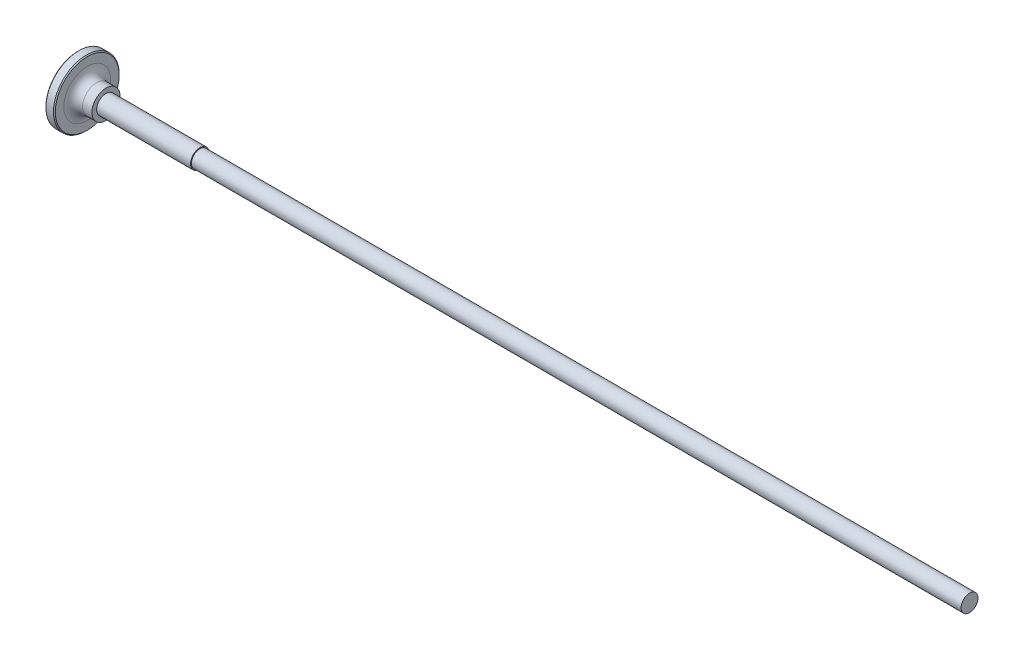
SolidWorks part; units mm, degrees
ref_plane "前视基准面" through (0, 0, 0) normal (0, 0, 1) x (1, 0, 0)
ref_plane "上视基准面" through (0, 0, 0) normal (0, 1, 0) x (1, 0, 0)
ref_plane "右视基准面" through (0, 0, 0) normal (1, 0, 0) x (0, 0, -1)
sketch "草图1" plane through (0, 0, 0) normal (1, 0, 0) x (0, 0, -1)
  circle A0 centre (0, 0) radius 35
  dimension "D1" = 70
extrude "凸台-拉伸1" add sketch "草图1" along normal blind 10
sketch "草图2" plane through (10, 0, 0) normal (1, 0, 0) x (0, 0, -1)
  circle A0 centre (0, 0) radius 15
  dimension "D1" = 30
extrude "凸台-拉伸2" add sketch "草图2" along normal blind 20
sketch "草图3" plane through (30, 0, 0) normal (1, 0, 0) x (0, 0, -1)
  circle A0 centre (0, 0) radius 10
  dimension "D1" = 20
extrude "凸台-拉伸3" add sketch "草图3" along normal blind 100
cosmetic thread "装饰螺纹线1" parameters "D1"=380, "D2"=19
sketch "草图4" plane through (130, 0, 0) normal (1, 0, 0) x (0, 0, -1)
  circle A0 centre (0, 0) radius 9
  dimension "D1" = 18
extrude "凸台-拉伸4" add sketch "草图4" along normal blind 820
chamfer "倒角1" distance 1 angle 45 2 edges at (0, 0, -35) (10, 0, -35)
fillet "圆角1" radius 10 1 edges at (10, 0, -15)
